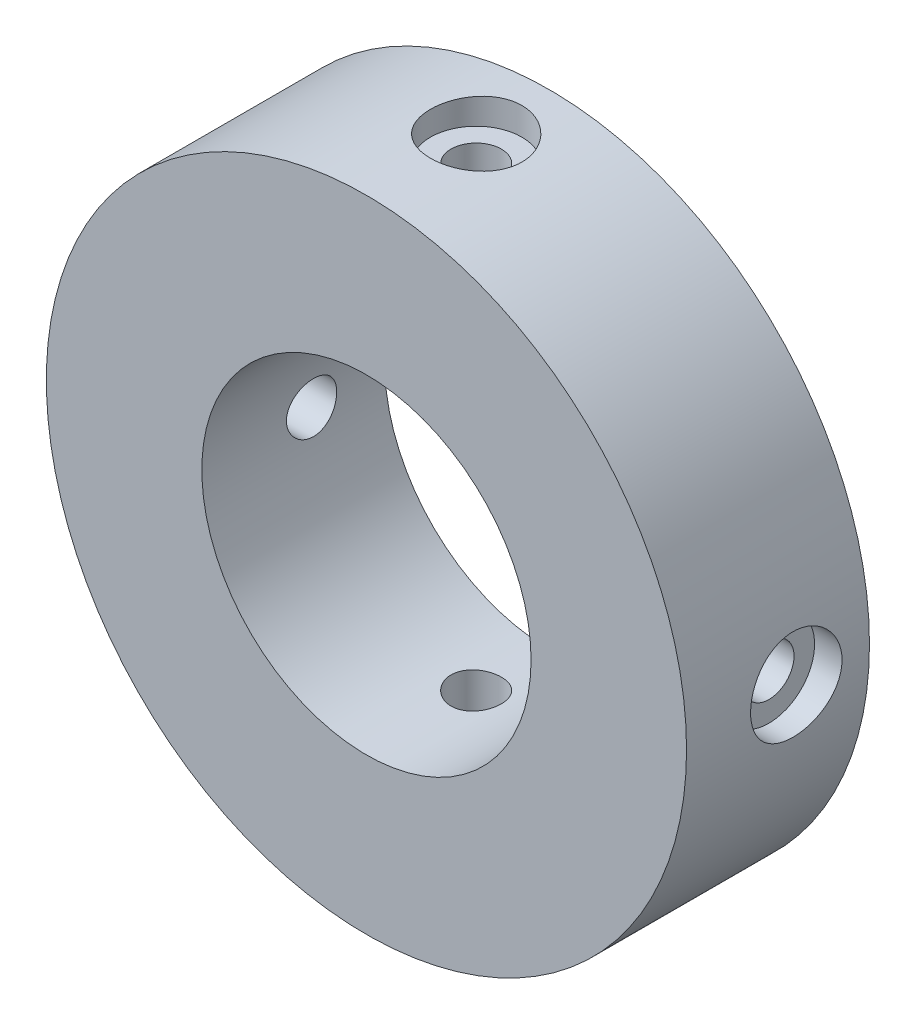
from build123d import *

# Parameters (mm, degrees)
SKETCH_1_R               = 35
SKETCH_1_R_2             = 18
EXTRUDE_1_DEPTH          = 20
SKETCH_5_R               = 2.75
CUT_EXTRUDE_1_DEPTH      = 33
CUT_EXTRUDE_START        = -32
SKETCH_6_R               = 5
CUT_EXTRUDE_3_DEPTH      = 33
PATTERN_CIRCULAR_1_COUNT = 4
PATTERN_CIRCULAR_2_COUNT = 4


with BuildPart() as part:
    # 草图1 → 凸台-拉伸1 (new body)
    with BuildSketch(Plane.XY):
        Circle(SKETCH_1_R)
        Circle(SKETCH_1_R_2, mode=Mode.SUBTRACT)
    extrude(amount=EXTRUDE_1_DEPTH)

    # 草图5 → 切除-拉伸1 (cut)
    with BuildSketch(Plane(origin=(0, 0, 0), x_dir=(1, 0, 0), z_dir=(0, 1, 0))):
        with Locations(Location((0, -8, 0), (0, 0, 270))):
            Circle(SKETCH_5_R)
    cut_extrude_1 = extrude(amount=-CUT_EXTRUDE_1_DEPTH, mode=Mode.SUBTRACT)

    # 草图6 → 切除-拉伸3 (cut)
    with BuildSketch(Plane(origin=(0, 0, 0), x_dir=(1, 0, 0), z_dir=(0, 1, 0)).offset(CUT_EXTRUDE_START)):
        with Locations(Location((0, -8, 0), (0, 0, 270))):
            Circle(SKETCH_6_R)
    cut_extrude_3 = extrude(amount=-CUT_EXTRUDE_3_DEPTH, mode=Mode.SUBTRACT)

    # 阵列(圆周)1: 切除-拉伸1, 切除-拉伸3 ×4 about axis
    pattern_circular_1_axis = Axis((0, 0, 0), (0, 0, 1))
    add([cut_extrude_1.rotate(pattern_circular_1_axis, i * 360 / PATTERN_CIRCULAR_1_COUNT) for i in range(1, PATTERN_CIRCULAR_1_COUNT)], mode=Mode.SUBTRACT)
    add([cut_extrude_3.rotate(pattern_circular_1_axis, i * 360 / PATTERN_CIRCULAR_1_COUNT) for i in range(1, PATTERN_CIRCULAR_1_COUNT)], mode=Mode.SUBTRACT)

    # 草图7 → M4x0.7 螺纹孔1 (revolve, cut)
    with BuildSketch(Plane(origin=(21.213203436, 21.213203436, 0), x_dir=(0, 1, 0), z_dir=(1, 0, 0))):
        Polygon((0, 0), (0, 11.091420021), (1.65, 10.1), (1.65, 0), align=None)
    m4x0_7_1 = revolve(axis=Axis((21.213203436, 21.213203436, -6.35), (0, 0, 1)), mode=Mode.SUBTRACT)

    # 阵列(圆周)2: M4x0.7 螺纹孔1 ×4 about axis
    pattern_circular_2_axis = Axis((0, 0, 0), (0, 0, 1))
    for i in range(1, PATTERN_CIRCULAR_2_COUNT):
        add(m4x0_7_1.rotate(pattern_circular_2_axis, i * 360 / PATTERN_CIRCULAR_2_COUNT), mode=Mode.SUBTRACT)


solid = part.part
